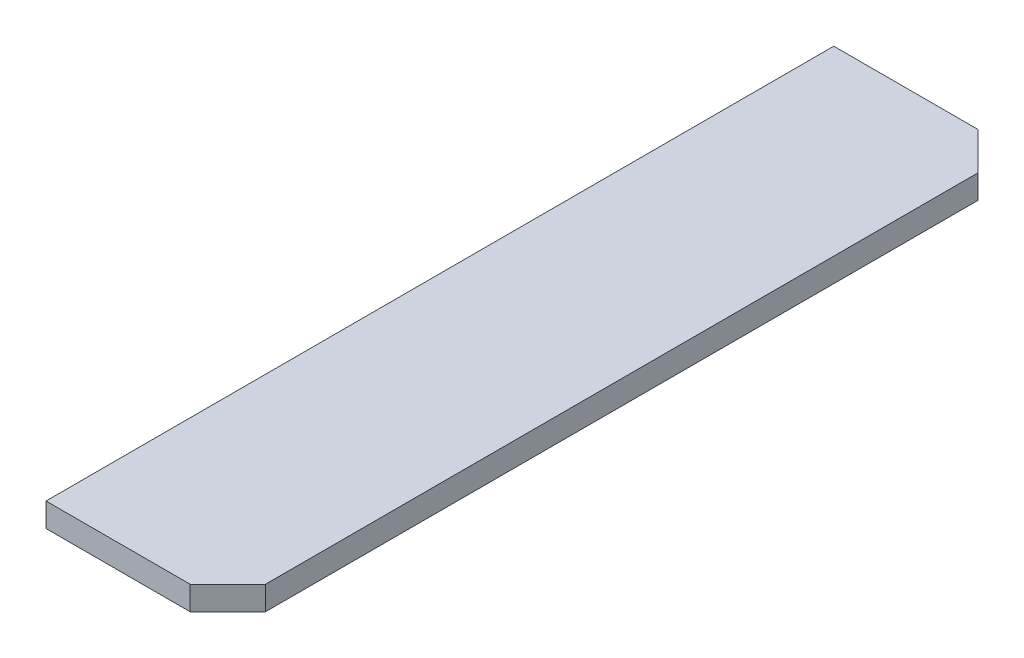
from build123d import *

# Parameters (mm, degrees)
BOSS_EXTRUDE1_DEPTH = 5


with BuildPart() as part:
    # Sketch3 → Boss-Extrude1 (new, symmetric)
    with BuildSketch(Plane(origin=(0, 0, 0), x_dir=(1, 0, 0), z_dir=(0, 1, 0))):
        Polygon((19.556, 140.716), (35.306, 124.966), (35.306, -173.734), (19.556, -189.484), (-40.894, -189.484), (-40.894, 140.716), align=None)
    extrude(amount=BOSS_EXTRUDE1_DEPTH, both=True)


solid = part.part
